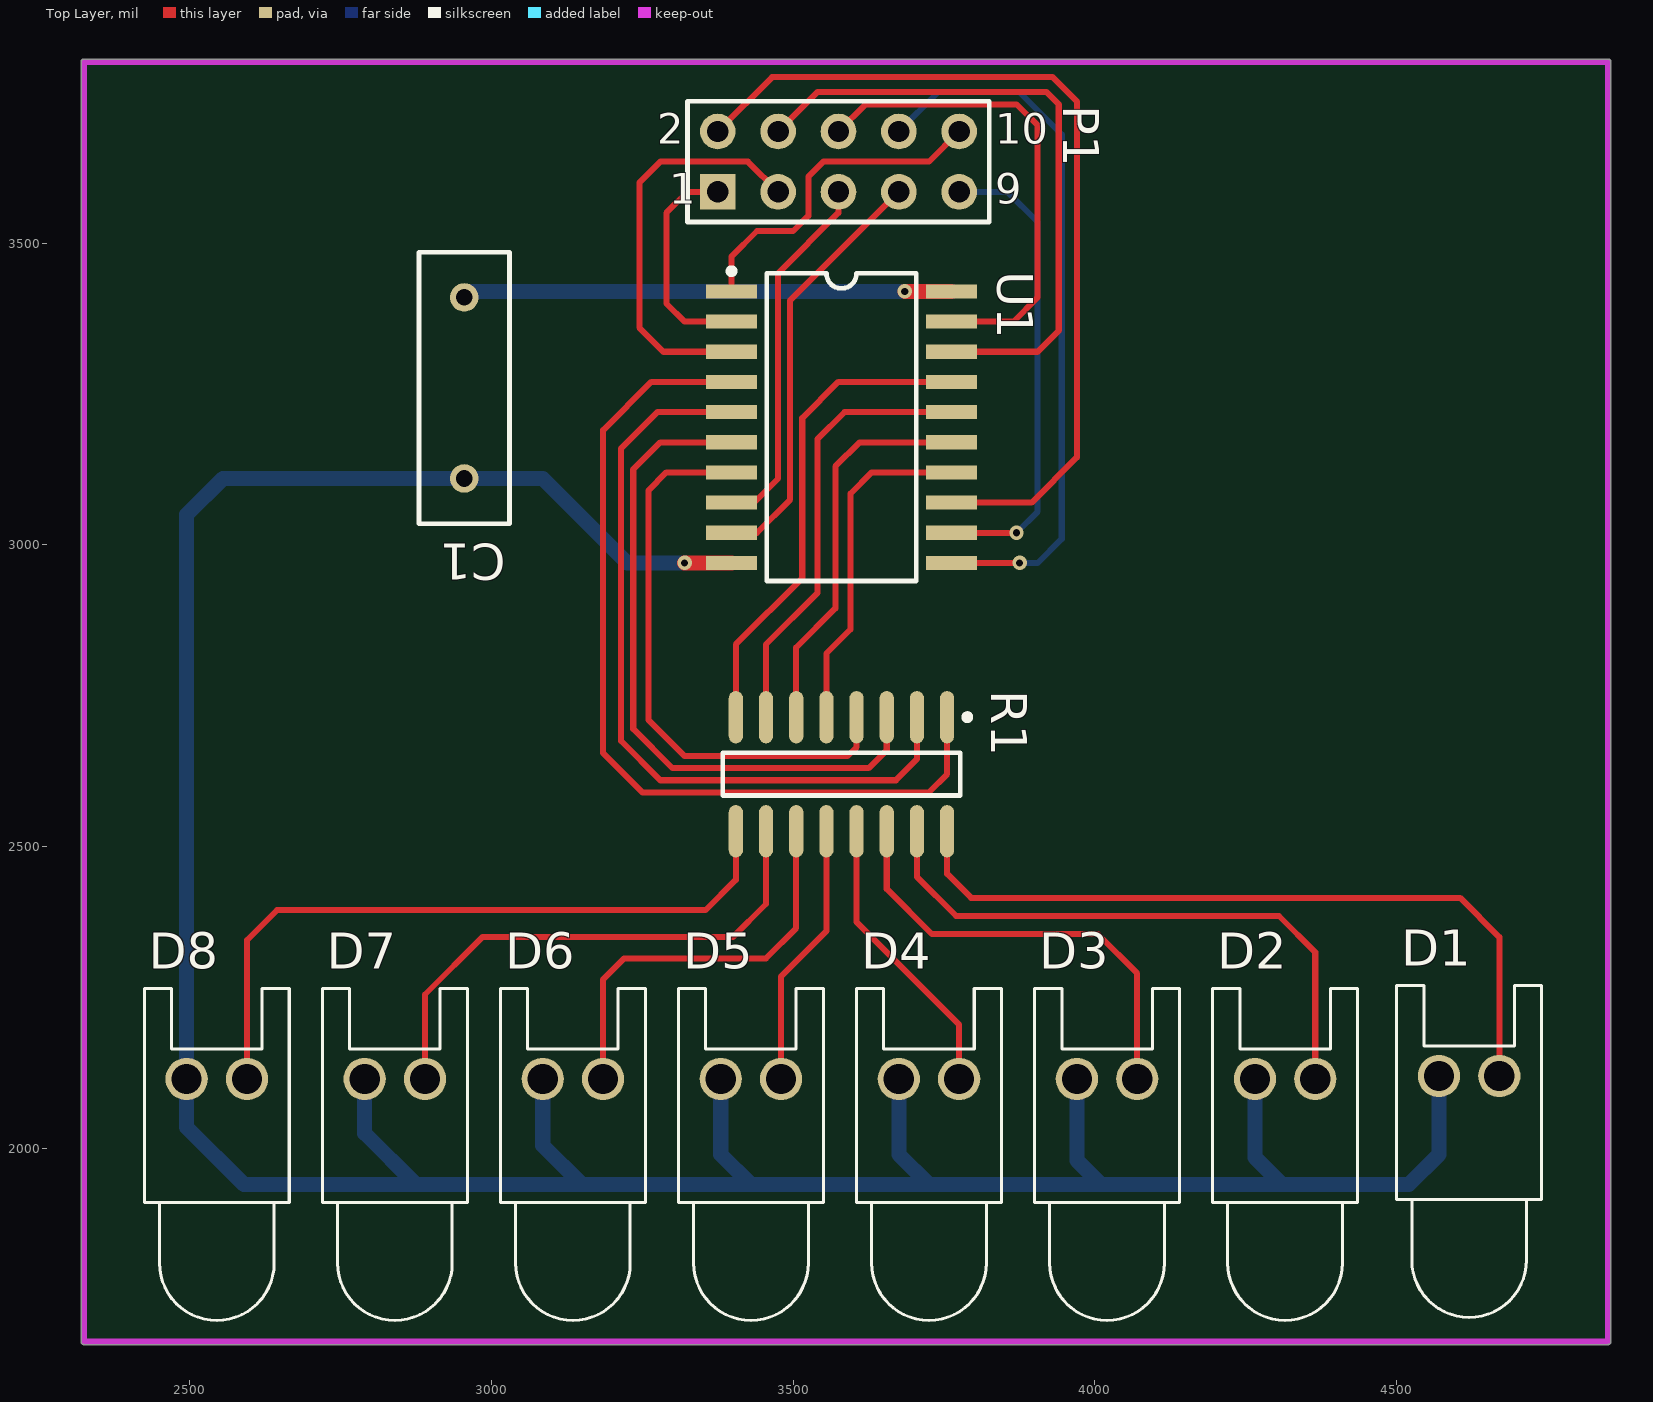
[diagram p0: Top Layer view]
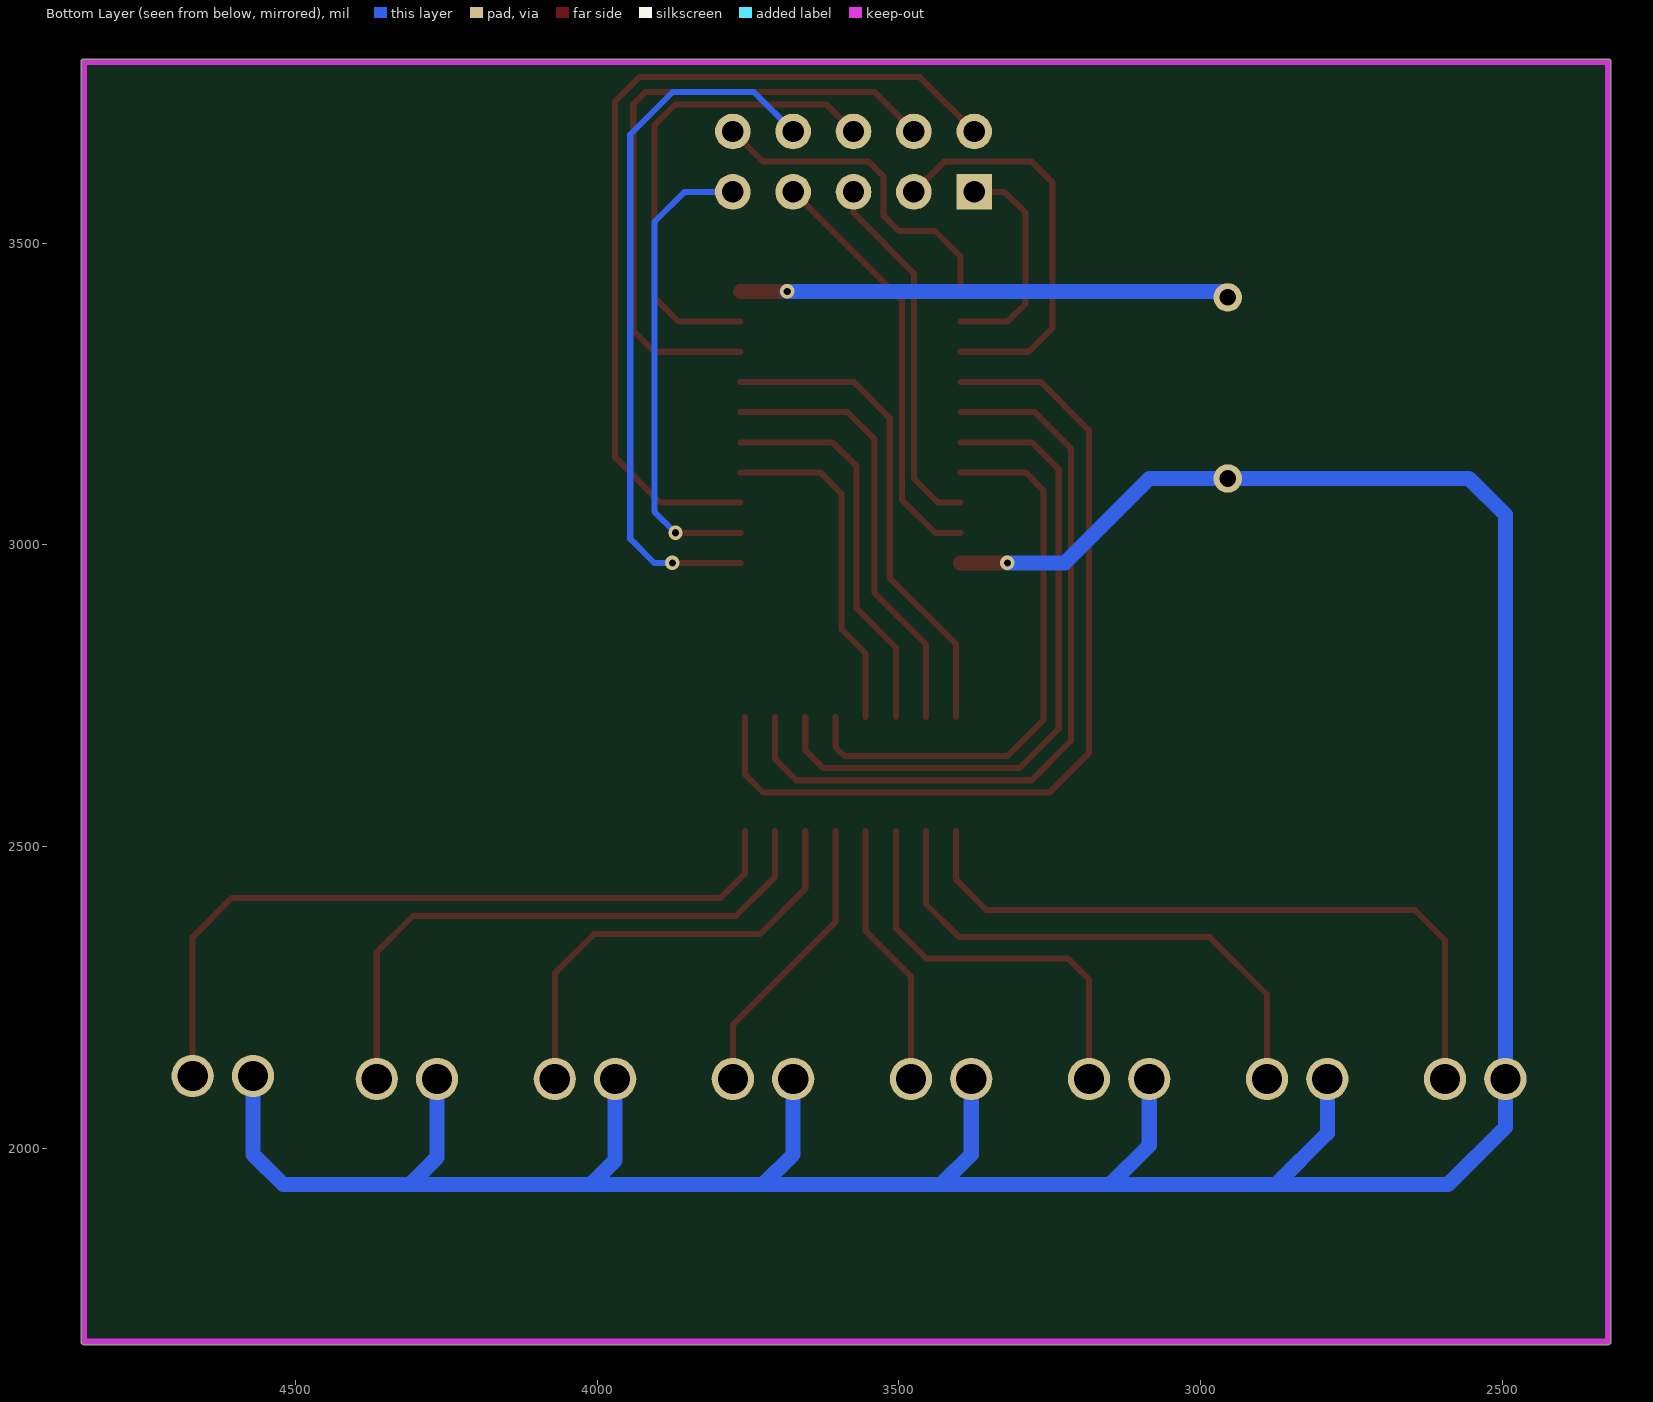
[diagram p1: Bottom Layer view, seen from below]
# Altium PCB MISC82900.PcbDoc
Units mil, origin at the board's own origin, x right, y up, seen from the top; angles counter-clockwise.
Board outline 2535.03 x 2130.03 mil, 2 copper layers (Top Layer, Bottom Layer); 12 components, 28 nets, 64 pads, 4 vias.

## Layer stack, top to bottom (the 12.6 mil dielectric is the usual default, probably not edited)
Top Solder: solder mask 0.4, Solder Resist, Dk 3.5
Top Layer: signal copper 1.4
Dielectric 1: dielectric 12.6, FR-4, Dk 4.8
Bottom Layer: signal copper 1.4
Bottom Solder: solder mask 0.4, Solder Resist, Dk 3.5

## Board outline
2319.99,1680 ccw(c2325,1680) 2325,1674.98 4850,1674.98 ccw(c4850,1680) 4855.02,1680 4855.02,3800 ccw(c4850,3800) 4850,3805.01 2325,3805.01 ccw(c2325,3800) 2319.99,3800

## Design rules (kind name [scope] priority, off if disabled: settings)
Clearance [All] p1: gap=10
MinimumSolderMaskSliver [All] p1: minsoldermaskwidth=0
PolygonConnect [All] p1: connectstyle=Relief reliefconductorwidth=10 reliefentries=4 polygonreliefangle="90 Angle" airgapwidth=10
RoutingVias [All] p1: holewidth=28 width=50 viastyle="Through Hole" minholewidth=28 minwidth=50 maxholewidth=28 maxwidth=50
SilkToSilkClearance [All] p1: silktosilkclearance=0
SilkToSolderMaskClearance [IsPad] p1: minsilkscreentomaskgap=0 clearancetoexposedcopper=TRUE
SolderMaskExpansion [All] p1: expansion=4
Width [All] p1: maxlimit=30 minlimit=10 preferedwidth=10
27 further rules are at their usual default settings.

## Components (designator, comment, footprint, x,y, rotation, side; value= is the part's Value field where it differs from the comment)
C1 "Cap" RAD-0.3 2955,3260 r270 top
D1 "LED0" LED-0 4620,2120 r0 top
D2 "LED0" LED-0 4315,2115 r0 top
D3 "LED0" LED-0 4020,2115 r0 top
D4 "LED0" LED-0 3725,2115 r0 top
D5 "LED0" LED-0 3430,2115 r0 top
D6 "LED0" LED-0 3135,2115 r0 top
D7 "LED0" LED-0 2840,2115 r0 top
D8 "LED0" LED-0 2545,2115 r0 top
P1 "Header 5X2" HDR2X5 3375,3585 r0 top
R1 "Res Pack3" SO-16_N 3580,2620 r270 top
U1 "TPIC6B273DW" DW020 3580,3195 r270 top

## Footprints (in the part's own frame and the unit in brackets; to place one, negate y for a bottom-side part, rotate by r counter-clockwise, add the part's x,y. Pads: shape width x height; smd on the part's side, far side on the other; paste and mask are expansions set on the pad)
DW020 [mm] "Plastic Small Outline; 20 Leads; Body Width 7.5 mm"
  rect 0.6x2.15 smd: 1(-5.715,-4.625) 2(-4.445,-4.625) 3(-3.175,-4.625) 4(-1.905,-4.625) 5(-0.635,-4.625) 6(0.635,-4.625) 7(1.905,-4.625) 8(3.175,-4.625) 9(4.445,-4.625) 10(5.715,-4.625) 11(5.715,4.625) 12(4.445,4.625) 13(3.175,4.625) 14(1.905,4.625) 15(0.635,4.625) 16(-0.635,4.625) 17(-1.905,4.625) 18(-3.175,4.625) 19(-4.445,4.625) 20(-5.715,4.625)
  silkscreen extent -6.69,-4.75 6.47,3.15
HDR2X5 [mm] "Connector; Header; 5x2 Position"
  rect 1.5x1.5 hole 0.9: 1(0,0)
  round 1.5 hole 0.9: 2(0,2.54) 3(2.54,0) 4(2.54,2.54) 5(5.08,0) 6(5.08,2.54) 7(7.62,0) 8(7.62,2.54) 9(10.16,0) 10(10.16,2.54)
  silkscreen extent -1.27,-1.27 11.43,3.81
LED-0 [mil] "LED; 2 Leads"
  round 70 hole 50: 1(50,0) 2(-50,0)
  silkscreen extent -120,-400 120,150
RAD-0.3 [mm] "Radial Cap, Thru-Hole; 2 Leads; 0.3 in Pin Spacing"
  round 1.2 hole 0.7: 1(-3.81,0) 2(3.81,0)
  silkscreen extent -5.71,-1.91 5.71,1.91
SO-16_N [mm] "SOIC, 16-Leads, Body 9.9x3.9mm, Pitch 1.27mm, IPC Medium Density"
  oval 2.2x0.6 smd: 1(-2.4,4.445) 2(-2.4,3.175) 3(-2.4,1.905) 4(-2.4,0.635) 5(-2.4,-0.635) 6(-2.4,-1.905) 7(-2.4,-3.175) 8(-2.4,-4.445) 9(2.4,-4.445) 10(2.4,-3.175) 11(2.4,-1.905) 12(2.4,-0.635) 13(2.4,0.635) 14(2.4,1.905) 15(2.4,3.175) 16(2.4,4.445)
  silkscreen extent -2.52,-5 0.9,5.42, body extent -2,-5 2,5, height 1.75

## Part data
C1: "Capacitor"
D1 D2 D3 D4 D5 D6 D7 D8: "Typical INFRARED GaAs LED"
P1: "Header, 5-Pin, Dual row"
R1: "Isolated Resistor Network"
U1: "Power Logic Octal D-Type Latch"

## Via types
v1: diameter 24, hole 12, Top Layer to Bottom Layer, 4 vias

## Nets (pads, with @x,y where several pads share a name; then routed paths per layer and width w, separated by ;. In a path a pad name is that pad's centre, name@x,y a point inside that pad or via, vN(x,y) a via of type N, cw(c..) or ccw(c..) an arc to the next point about the centre after c; other vN are vias at no path point)
CLK: P1.8 U1.11 | length 1195.4
  Top Layer w10: U1.11 v1(3875,2970)
  Bottom Layer w10: P1.8 3740,3750 3875,3750 3945,3680 3945,3010 3905,2970 v1(3875,2970)
CLR: P1.10 U1.1 | length 558.9
  Top Layer w10: U1.1 3397.91,3477.91 3440,3520 3500,3520 3525,3545 3525,3610 3550,3635 3725,3635 P1.10
DATA0: P1.1 U1.2 | length 369.8
  Top Layer w10: P1.1 3325,3585 3290,3550 3290,3400 3320,3370 U1.2
DATA1: P1.3 U1.3 | length 674.7
  Top Layer w10: U1.3 3285,3320 3245,3360 3245,3600 3280,3635 3425,3635 P1.3
DATA2: P1.5 U1.8 | length 610.1
  Top Layer w10: U1.8 3435,3070 3475,3110 3475,3450 3575,3550 P1.5
DATA3: P1.7 U1.9 | length 704.4
  Top Layer w10: U1.9 3440,3020 3495,3075 3495,3405 P1.7
DATA4: P1.9 U1.12 | length 788.1
  Top Layer w10: U1.12 v1(3870,3020)
  Bottom Layer w10: P1.9 3855,3585 3905,3535 3905,3055 v1(3870,3020)
DATA5: P1.2 U1.13 | length 1477.8
  Top Layer w10: P1.2 3465,3775 3930,3775 3970,3735 3970,3145 3895,3070 U1.13
DATA6: P1.4 U1.18 | length 1067.6
  Top Layer w10: P1.4 3540,3750 3920,3750 3940,3730 3940,3355 3905,3320 U1.18
DATA7: P1.6 U1.19 | length 807.6
  Top Layer w10: P1.6 3620,3730 3870,3730 3905,3695 3905,3410 3865,3370 U1.19
GND: C1.2 D1.2 D2.2 D3.2 D4.2 D5.2 D6.2 D7.2 D8.2 U1.10 | length 5454.6
  Top Layer w25: v1(3320,2970) U1.10
  Bottom Layer w25: D7.2 2790,2025 2875,1940 ; D6.2 3085,2005 3150,1940 ; v1(3320,2970) 3225,2970 3085,3110 C1.2 2555,3110 2495,3050 D8.2 2495,2035 2590,1940 2875,1940 ; D5.2 3380,1990 3430,1940 ; D4.2 3675,1990 3725,1940 ; D3.2 3970,1980 4010,1940 ; D2.2 4265,1985 4310,1940 ; D1.2 4570,1990 4520,1940 4310,1940 ; 2875,1940 3150,1940 ; 3150,1940 3430,1940 ; 3430,1940 3725,1940 ; 3725,1940 4010,1940 ; 4010,1940 4310,1940
NetD1_1: D1.1 R1.16 | length 1259
  Top Layer w10: R1.16 3755,2455 3795,2415 4605,2415 4670,2350 D1.1
NetD2_1: D2.1 R1.15 | length 997.3
  Top Layer w10: R1.15 3705,2450 3770,2385 4305,2385 4365,2325 D2.1
NetD3_1: D3.1 R1.14 | length 743.5
  Top Layer w10: R1.14 3655,2430 3730,2355 4005,2355 4070,2290 D3.1
NetD4_1: D4.1 R1.13 | length 480.9
  Top Layer w10: R1.13 3605,2375 3775,2205 D4.1
NetD5_1: D5.1 R1.12 | length 441.6
  Top Layer w10: D5.1 3480,2285 3555,2360 R1.12
NetD6_1: D6.1 R1.11 | length 680.7
  Top Layer w10: D6.1 3185,2280 3220,2315 3455,2315 3505,2365 R1.11
NetD7_1: D7.1 R1.10 | length 887.6
  Top Layer w10: D7.1 2890,2255 2985,2350 3400,2350 3455,2405 R1.10
NetD8_1: D8.1 R1.9 | length 1161.9
  Top Layer w10: D8.1 2595,2345 2645,2395 3355,2395 3405,2445 R1.9
NetR1_1: R1.1 U1.4 | length 1484.9
  Top Layer w10: U1.4 3265,3270 3185,3190 3185,2655 3250,2590 3725,2590 3755,2620 R1.1
NetR1_2: R1.2 U1.5 | length 1293.7
  Top Layer w10: U1.5 3275,3220 3215,3160 3215,2675 3280,2610 3670,2610 3705,2645 R1.2
NetR1_3: R1.3 U1.6 | length 1125.4
  Top Layer w10: U1.6 3280,3170 3235,3125 3235,2695 3300,2630 3625,2630 3655,2660 R1.3
NetR1_4: R1.4 U1.7 | length 955.9
  Top Layer w10: U1.7 3290,3120 3260,3090 3260,2710 3320,2650 3590,2650 3605,2665 R1.4
NetR1_5: R1.5 U1.14 | length 568.7
  Top Layer w10: R1.5 3555,2820 3595,2860 3595,3085 3630,3120 U1.14
NetR1_6: R1.6 U1.15 | length 651.1
  Top Layer w10: R1.6 3505,2830 3570,2895 3570,3130 3610,3170 U1.15
NetR1_7: R1.7 U1.16 | length 736.4
  Top Layer w10: R1.7 3455,2835 3540,2920 3540,3175 3585,3220 U1.16
NetR1_8: R1.8 U1.17 | length 813
  Top Layer w10: R1.8 3405,2835 3515,2945 3515,3210 3575,3270 U1.17
VCC: C1.1 U1.20 | length 811.2
  Top Layer w25: v1(3685,3420) U1.20
  Bottom Layer w25: C1.1 2965,3420 v1(3685,3420)

## Keep-outs
Keep-Out Layer:
  lines w10: 2425,3800 4850,3800 4850,1680 2445,1680 2325,1680 2325,3800 2445,3800